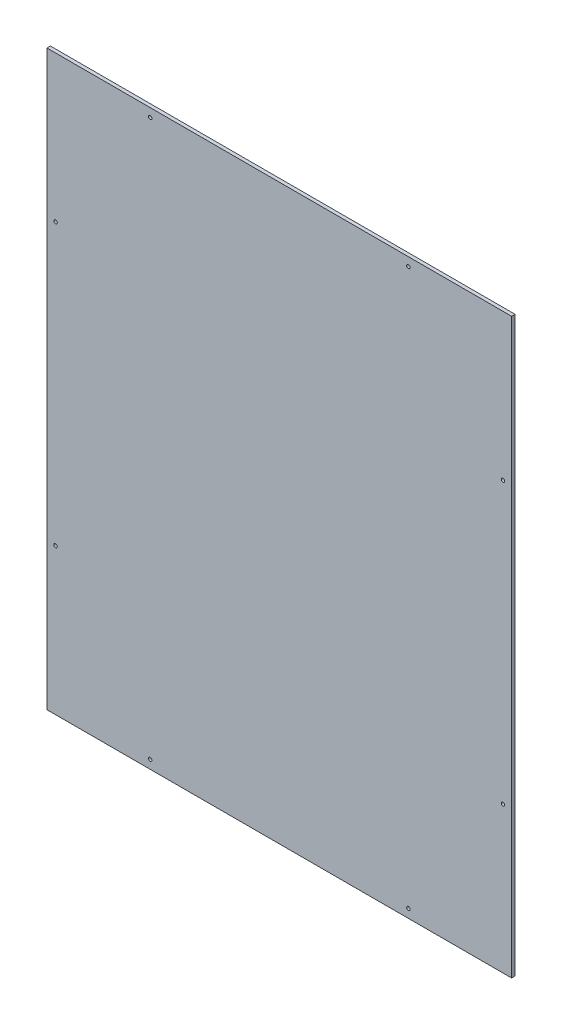
from build123d import *

# Parameters (mm, degrees)
SKETCH_1_W            = 540
SKETCH_1_H            = 666
EXTRUDE_1_DEPTH       = 2
HOLE_WIZARD_4_0_4_1_D = 4
HOLE_WIZARD_4_0_4_2_D = 4


with BuildPart() as part:
    # 草图1 → 凸台-拉伸1 (new, symmetric)
    with BuildSketch(Plane.XY):
        Rectangle(SKETCH_1_W, SKETCH_1_H)
    extrude(amount=EXTRUDE_1_DEPTH, both=True)

    # Ø4.0 (4) 直径孔1 (through all)
    with Locations(Plane(origin=(0, 0, -2), x_dir=(-1, 0, 0), z_dir=(0, 0, -1))):
        with Locations((-260, 163), (-260, -163)):
            hole_wizard_4_0_4_1 = Hole(HOLE_WIZARD_4_0_4_1_D / 2)

    # Ø4.0 (4) 直径孔2 (through all)
    with Locations(Plane(origin=(0, 0, -2), x_dir=(-1, 0, 0), z_dir=(0, 0, -1))):
        with Locations((-150, 323), (150, 323)):
            hole_wizard_4_0_4_2 = Hole(HOLE_WIZARD_4_0_4_2_D / 2)

    # 镜向1: Ø4.0 (4) 直径孔2 across plane
    add(hole_wizard_4_0_4_2.mirror(Plane.ZX), mode=Mode.SUBTRACT)

    # 镜向2: Ø4.0 (4) 直径孔1 across plane
    add(hole_wizard_4_0_4_1.mirror(Plane(origin=(0, 0, 0), x_dir=(0, 0, 1), z_dir=(1, 0, 0))), mode=Mode.SUBTRACT)


solid = part.part
